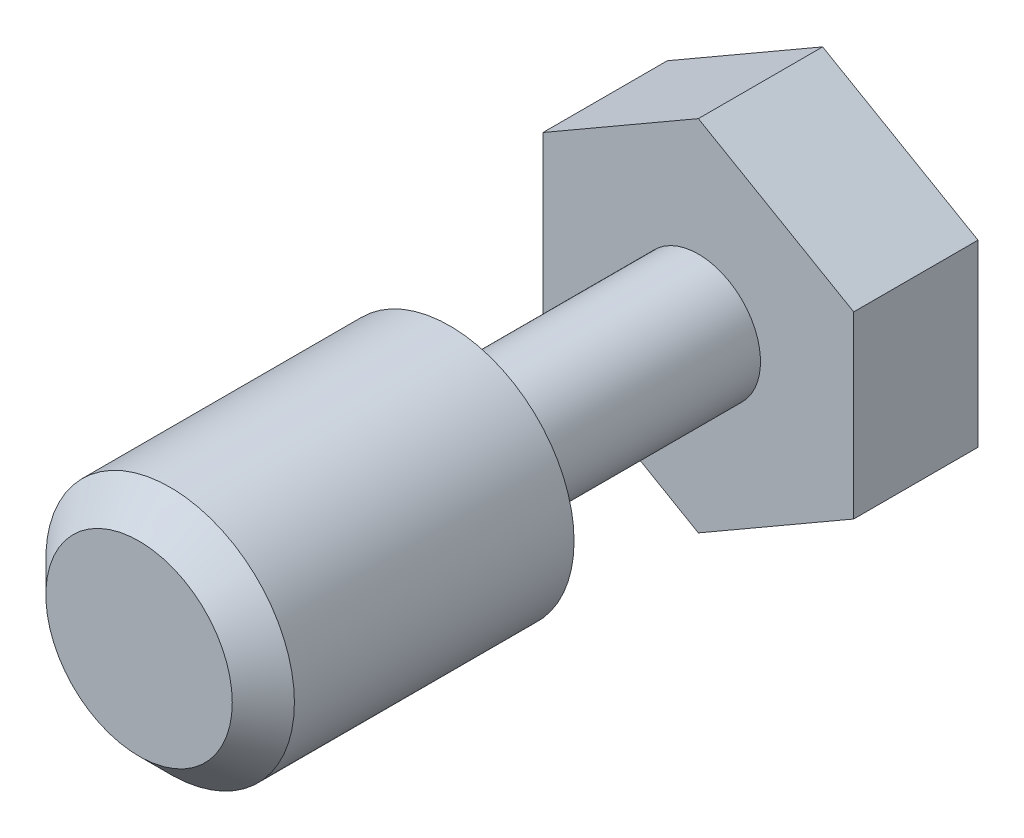
from build123d import *

# Parameters (mm, degrees)
SKETCH1_R           = 2
BOSS_EXTRUDE1_DEPTH = 5
SKETCH2_R           = 1
BOSS_EXTRUDE2_DEPTH = 4
BOSS_EXTRUDE3_DEPTH = 2
CHAMFER1_SIZE       = 0.5


with BuildPart() as part:
    # Sketch1 → Boss-Extrude1 (new body)
    with BuildSketch(Plane.XY):
        Circle(SKETCH1_R)
    extrude(amount=BOSS_EXTRUDE1_DEPTH)

    # Sketch2 → Boss-Extrude2 (add)
    with BuildSketch(Plane(origin=(0, 0, 0), x_dir=(-1, 0, 0), z_dir=(0, 0, -1))):
        Circle(SKETCH2_R)
    extrude(amount=BOSS_EXTRUDE2_DEPTH)

    # Sketch3 → Boss-Extrude3 (add)
    with BuildSketch(Plane(origin=(0, 0, -4), x_dir=(-1, 0, 0), z_dir=(0, 0, -1))):
        Polygon((0, 2.886751346), (-2.5, 1.443375673), (-2.5, -1.443375673), (0, -2.886751346), (2.5, -1.443375673), (2.5, 1.443375673), align=None)
    extrude(amount=BOSS_EXTRUDE3_DEPTH)

    # Chamfer1
    chamfer1_edges = [part.edges().sort_by_distance(p)[0] for p in [
        (-2, 0, 5),
    ]]
    chamfer(chamfer1_edges, length=CHAMFER1_SIZE)


solid = part.part
